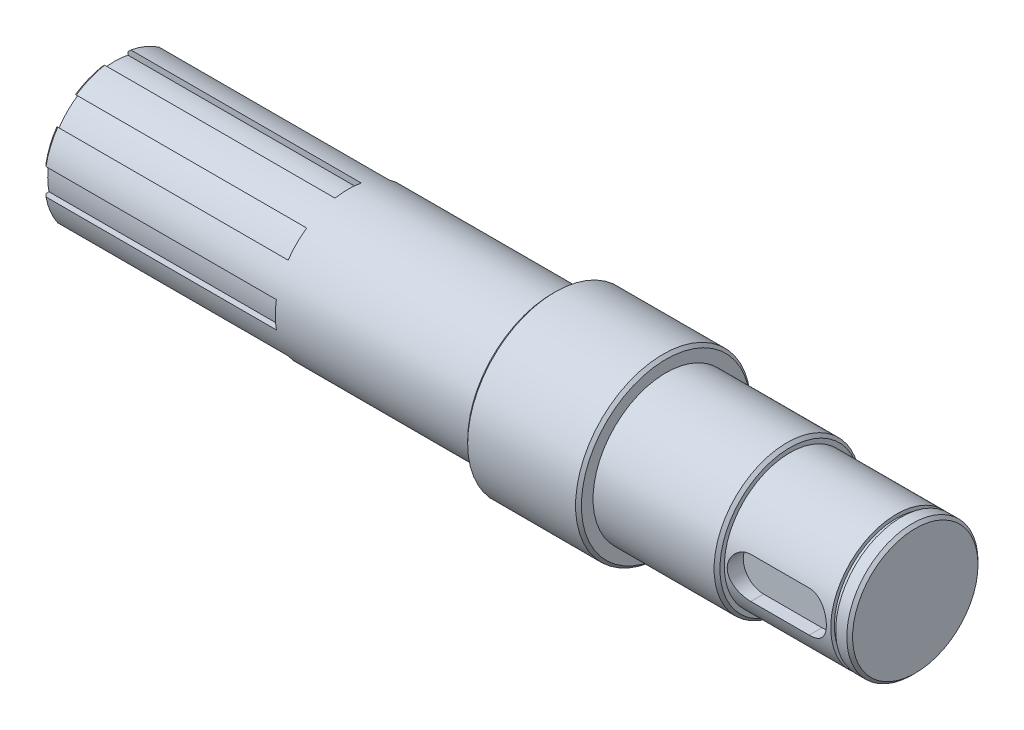
SolidWorks part; units mm, degrees
ref_plane "前视基准面" through (0, 0, 0) normal (0, 0, 1) x (1, 0, 0)
ref_plane "上视基准面" through (0, 0, 0) normal (0, 1, 0) x (1, 0, 0)
ref_plane "右视基准面" through (0, 0, 0) normal (1, 0, 0) x (0, 0, -1)
sketch "草图1" plane through (0, 0, 0) normal (0, 0, 1) x (1, 0, 0)
  line L0 (0, 0) -> (319.6501, 0) construction
  line L1 (0, 0) -> (0, 130.0325) construction
  line L2 (0, 0) -> (0, 25)
  line L3 (0, 25) -> (150, 25)
  line L4 (231.5, 25) -> (231.5, 22.5)
  line L5 (231.5, 22.5) -> (274.5, 22.5)
  line L6 (274.5, 22.5) -> (274.5, 0)
  line L7 (274.5, 0) -> (0, 0)
  line L8 (150, 25) -> (150, 30)
  line L9 (150, 30) -> (189, 30)
  line L10 (189, 30) -> (189, 25)
  line L11 (189, 25) -> (231.5, 25)
  dimension "D1" = 50
  dimension "D2" = 42.5
  dimension "D3" = 45
  dimension "D4" = 43
  dimension "D5" = 60
  dimension "D6" = 39
  dimension "D7" = 150
revolve "旋转1" add sketch "草图1" angle 360 about L7
chamfer "倒角1" distance 1 angle 45 4 edges at (274.5, 0, -22.5) (231.5, 0, -25) (189, 0, -30) (150, 0, -30)
ref_plane "基准面1" through (268, 0, 0) normal (1, 0, 0) x (0, 0, -1)
sketch "草图2" plane through (268, 0, 0) normal (1, 0, 0) x (0, 0, -1)
  circle A0 centre (0, 0) radius 21.25
  circle A1 centre (0, 0) radius 22.5
  dimension "D1" = 45
  dimension "D2" = 42.5
extrude "切除-拉伸1" cut sketch "草图2" along normal blind 1.7
ref_plane "基准面2" through (0, 0, 22.5) normal (0, 0, 1) x (1, 0, 0)
sketch "草图3" plane through (0, 0, 22.5) normal (0, 0, 1) x (1, 0, 0)
  line L0 (0, 0) -> (272.7051, 0) construction
  line L1 (239.5, 0) -> (259.5, 0) construction
  line L2 (239.5, 7) -> (259.5, 7)
  line L3 (239.5, -7) -> (259.5, -7)
  line L5 (274.5, -21.5) -> (274.5, 21.5) construction
  arc A0 (239.5, 7) -> (239.5, -7) centre (239.5, 0) ccw
  arc A1 (259.5, -7) -> (259.5, 7) centre (259.5, 0) ccw
  point P5 (249.5, 0)
  point P11 (266.5, 0)
  dimension "D2" = 20
  dimension "D1" = 14
  dimension "D3" = 8
extrude "切除-拉伸2" cut sketch "草图3" against normal blind 5.5
sketch "草图4" plane through (0, 0, 0) normal (-1, 0, 0) x (0, 0, 1)
  line L0 (0, 0) -> (0, 33.8685) construction
  line L1 (0, 0) -> (38.9741, 0) construction
  line L2 (-4.5, 24.5917) -> (-4.5, 22.5555)
  line L3 (4.5, 24.5917) -> (4.5, 22.5555)
  line L4 (20.5709, 14.207) -> (19.1311, 12.7672)
  line L5 (14.207, 20.5709) -> (12.7672, 19.1311)
  line L6 (24.5917, -4.5) -> (22.5555, -4.5)
  line L7 (24.5917, 4.5) -> (22.5555, 4.5)
  line L8 (14.207, -20.5709) -> (12.7672, -19.1311)
  line L9 (20.5709, -14.207) -> (19.1311, -12.7672)
  line L10 (-4.5, -24.5917) -> (-4.5, -22.5555)
  line L11 (4.5, -24.5917) -> (4.5, -22.5555)
  line L12 (-20.5709, -14.207) -> (-19.1311, -12.7672)
  line L13 (-14.207, -20.5709) -> (-12.7672, -19.1311)
  line L14 (-24.5917, 4.5) -> (-22.5555, 4.5)
  line L15 (-24.5917, -4.5) -> (-22.5555, -4.5)
  line L16 (-14.207, 20.5709) -> (-12.7672, 19.1311)
  line L17 (-20.5709, 14.207) -> (-19.1311, 12.7672)
  arc A0 (-12.7672, 19.1311) -> (-19.1311, 12.7672) centre (0, 0) ccw
  arc A1 (-14.207, 20.5709) -> (-20.5709, 14.207) centre (0, 0) ccw
  arc A2 (4.5, 22.5555) -> (-4.5, 22.5555) centre (0, 0) ccw
  arc A3 (4.5, 24.5917) -> (-4.5, 24.5917) centre (0, 0) ccw
  arc A4 (19.1311, 12.7672) -> (12.7672, 19.1311) centre (0, 0) ccw
  arc A5 (20.5709, 14.207) -> (14.207, 20.5709) centre (0, 0) ccw
  arc A6 (22.5555, -4.5) -> (22.5555, 4.5) centre (0, 0) ccw
  arc A7 (24.5917, -4.5) -> (24.5917, 4.5) centre (0, 0) ccw
  arc A8 (12.7672, -19.1311) -> (19.1311, -12.7672) centre (0, 0) ccw
  arc A9 (14.207, -20.5709) -> (20.5709, -14.207) centre (0, 0) ccw
  arc A10 (-4.5, -22.5555) -> (4.5, -22.5555) centre (0, 0) ccw
  arc A11 (-4.5, -24.5917) -> (4.5, -24.5917) centre (0, 0) ccw
  arc A12 (-19.1311, -12.7672) -> (-12.7672, -19.1311) centre (0, 0) ccw
  arc A13 (-20.5709, -14.207) -> (-14.207, -20.5709) centre (0, 0) ccw
  arc A14 (-22.5555, 4.5) -> (-22.5555, -4.5) centre (0, 0) ccw
  arc A15 (-24.5917, 4.5) -> (-24.5917, -4.5) centre (0, 0) ccw
  point P41 (0, 0)
  dimension "D1" = 46
  dimension "D2" = 50
  dimension "D3" = 9
  dimension "D4" = 8
extrude "切除-拉伸3" cut sketch "草图4" against normal blind 80
chamfer "倒角2" distance 1 angle 45 8 edges at (0, 23.097, -9.5671) (0, 9.5671, -23.097) (0, -9.5671, -23.097) (0, -23.097, -9.5671) (0, -23.097, 9.5671) (0, -9.5671, 23.097) (0, 9.5671, 23.097) (0, 23.097, 9.5671)
